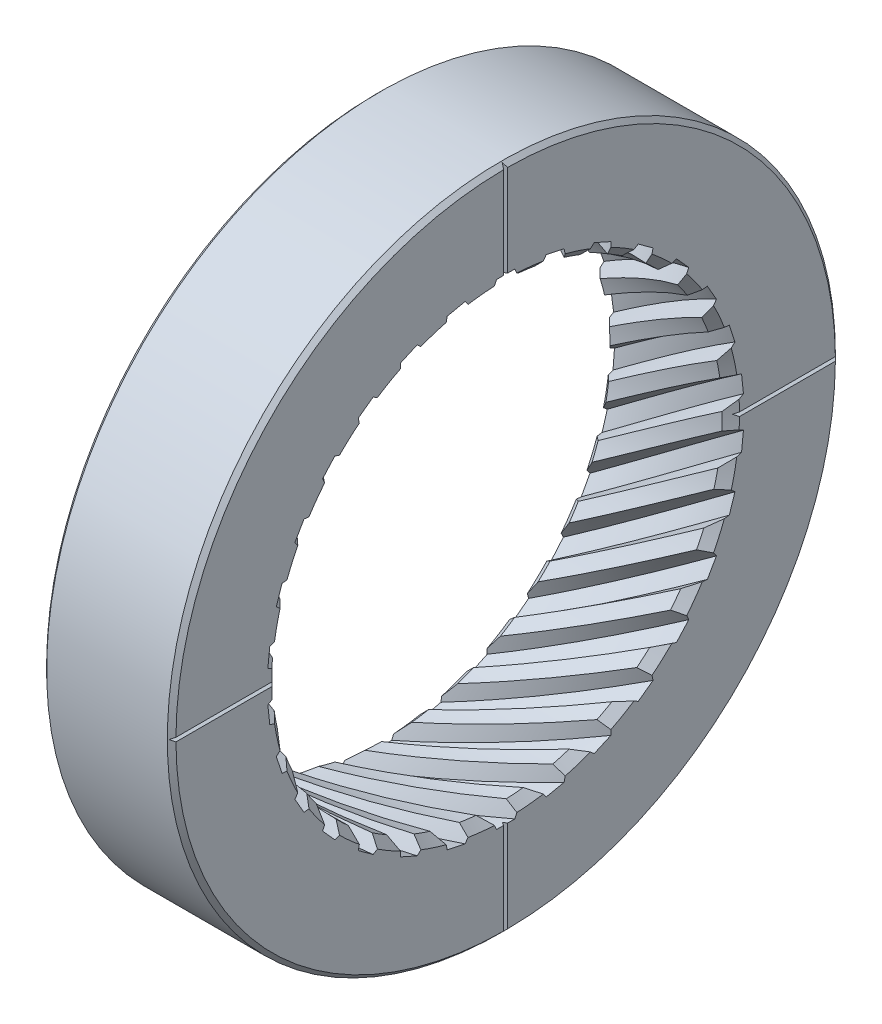
SolidWorks part; units mm, degrees
material "45"
ref_plane "前视基准面" through (0, 0, 0) normal (0, 0, 1) x (1, 0, 0)
ref_plane "上视基准面" through (0, 0, 0) normal (0, 1, 0) x (1, 0, 0)
ref_plane "右视基准面" through (0, 0, 0) normal (1, 0, 0) x (0, 0, -1)
sketch "草图1" plane through (0, 0, 0) normal (1, 0, 0) x (0, 0, -1)
  circle A0 centre (0, 0) radius 77.5
  circle A1 centre (0, 0) radius 52.25
  dimension "D1" = 155
  dimension "D2" = 104.5
extrude "凸台-拉伸1" add sketch "草图1" along normal blind 30
chamfer "倒角2" distance 2 angle 45 2 edges at (0, 0, -52.25) (30, 0, -52.25)
sketch "草图2" plane through (30, 0, 0) normal (1, 0, 0) x (0, 0, -1)
  circle A1 centre (0, 0) radius 53.5
  circle A2 centre (0, 0) radius 52.25 construction
  dimension "D1" = 107
curve "螺旋线/涡状线1" pitch 480 height 30 turns 0.0625
sketch "扫描点" plane through (30, 0, 0) normal (1, 0, 0) x (0, 0, -1)
  line L0 (0, -1000) -> (0, 49000) construction
  line L1 (-2.9, 53.5) -> (2.9, 53.5) construction
  line L2 (-2.1208, 55.25) -> (-3.6792, 51.75)
  line L3 (2.1208, 55.25) -> (3.6792, 51.75)
  line L4 (-2.1208, 55.25) -> (2.1208, 55.25)
  line L5 (-3.6792, 51.75) -> (3.6792, 51.75)
  spline S0 degree 3 poles (0, 53.5) (2.3338, 53.5) (7.0034, 53.194) (13.8861, 51.8249) (18.3174, 50.3207) (20.4736, 49.4276) knots 0 0 0 0 0.333333 0.666667 1 1 1 1 construction
  point P0 (0, 53.5)
  dimension "D1" = 5.8
  dimension "D2" = 48
  dimension "D3" = 3.5
chamfer "倒角1" distance 1 angle 45 2 edges at (0, 0, -77.5) (30, 0, -77.5)
sweep "切除-扫描3" cut profiles "扫描点" path "螺旋线/涡状线1"
pattern_circular "阵列(圆周)4" count 30 over 360 about axis through (30, 0, 0) along (-1, 0, 0) of "切除-扫描3"
sketch "检测图" plane through (30, 0, 0) normal (1, 0, 0) x (0, 0, -1)
  line L0 (-2.5937, 54.188) -> (-2.1208, 55.25) construction
  line L1 (2.1208, 55.25) -> (2.5937, 54.188) construction
  line L2 (8.7293, 53.5431) -> (9.4126, 54.4836) construction
  circle A0 centre (0, 0) radius 53.5
  point P3 (-2.9359, 53.4194)
  point P4 (2.9359, 53.4194)
  point P7 (8.2348, 52.8624)
  dimension "D1" = 107
sketch "轨迹点" plane through (30, 0, 0) normal (1, 0, 0) x (0, 0, -1)
  line L0 (0, 0) -> (0, 134.2706) construction
  line L1 (0, 0) -> (14.6275, 139.1715) construction
  point P2 (5.5923, 53.2069)
  dimension "D1" = 6
  dimension "D2" = 53.5
ref_plane "基准面1" through (0, 77.5, 0) normal (0, 1, 0) x (1, 0, 0)
sketch "草图6" plane through (0, 77.5, 0) normal (0, 1, 0) x (1, 0, 0)
  line L0 (-1000, 0) -> (49000, 0) construction
  line L1 (0, 76.5) -> (0, -76.5) construction
  line L2 (0.8, 0) -> (0, 0.4619)
  line L3 (0, 0.4619) -> (0, -0.4619)
  line L4 (0, -0.4619) -> (0.8, 0)
  line L5 (30, -76.5) -> (30, 76.5) construction
  line L6 (29.2, 0) -> (30, -0.4619)
  line L7 (30, -0.4619) -> (30, 0.4619)
  line L8 (30, 0.4619) -> (29.2, 0)
  circle A0 centre (0.2667, 0) radius 0.2667 construction
  circle A1 centre (29.7333, 0) radius 0.2667 construction
  dimension "D1" = 0.8
  dimension "D2" = 0.8
extrude "切除-拉伸2" cut sketch "草图6" against normal through all
pattern_circular "阵列(圆周)6" count 4 over 360 about axis through (30, 0, 0) along (-1, 0, 0) of "切除-拉伸2"
equation "\"XMMCDM\"= \"QC名称代码\""
